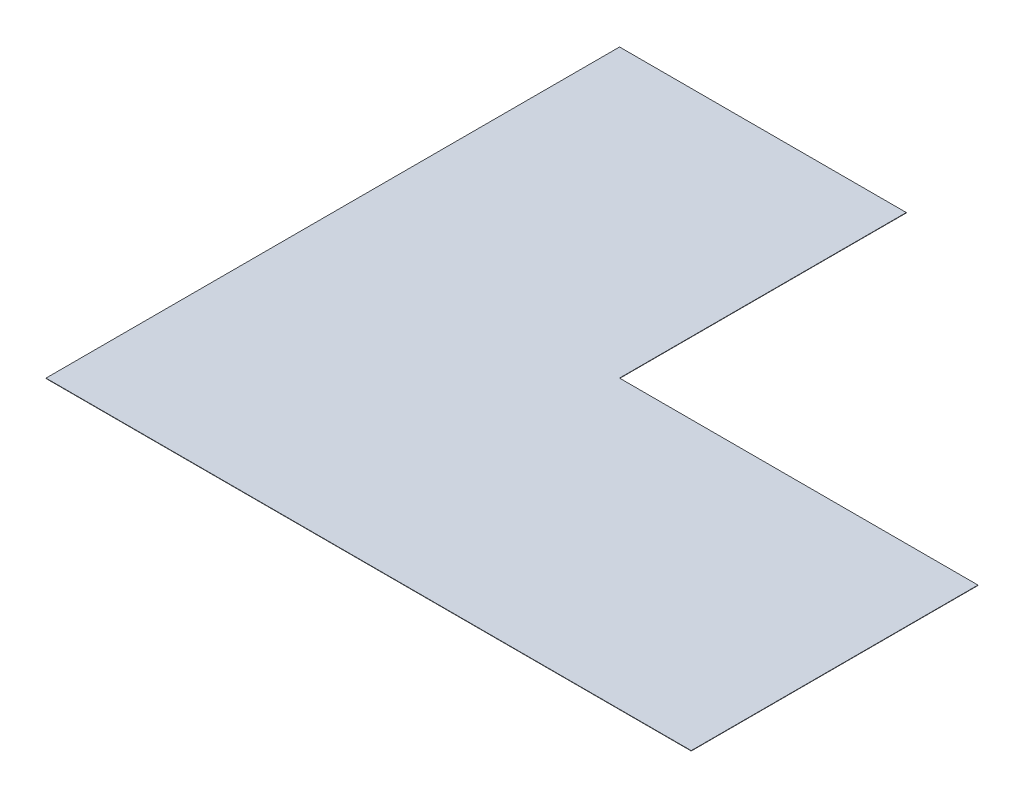
SolidWorks part; units mm, degrees
ref_plane "Front Plane" through (0, 0, 0) normal (0, 0, 1) x (1, 0, 0)
ref_plane "Top Plane" through (0, 0, 0) normal (0, 1, 0) x (1, 0, 0)
ref_plane "Right Plane" through (0, 0, 0) normal (1, 0, 0) x (0, 0, -1)
sketch "Sketch1" plane through (0, 0, 0) normal (0, 1, 0) x (1, 0, 0)
  line L1 (-900, -800) -> (900, -800)
  line L2 (-900, -800) -> (-900, 800)
  line L3 (-900, 800) -> (-100, 800)
  line L4 (900, -800) -> (900, 0)
  line L5 (-900, -800) -> (0, 0) construction
  line L6 (-900, 800) -> (900, -800) construction
  line L7 (0, 0) -> (900, 0)
  line L8 (-100, 800) -> (-100, 0)
  line L9 (-100, 0) -> (0, 0)
  point P0 (0, 0)
  dimension "D1" = 1800
  dimension "D2" = 1600
extrude "Boss-Extrude1" add sketch "Sketch1" along normal blind 1
